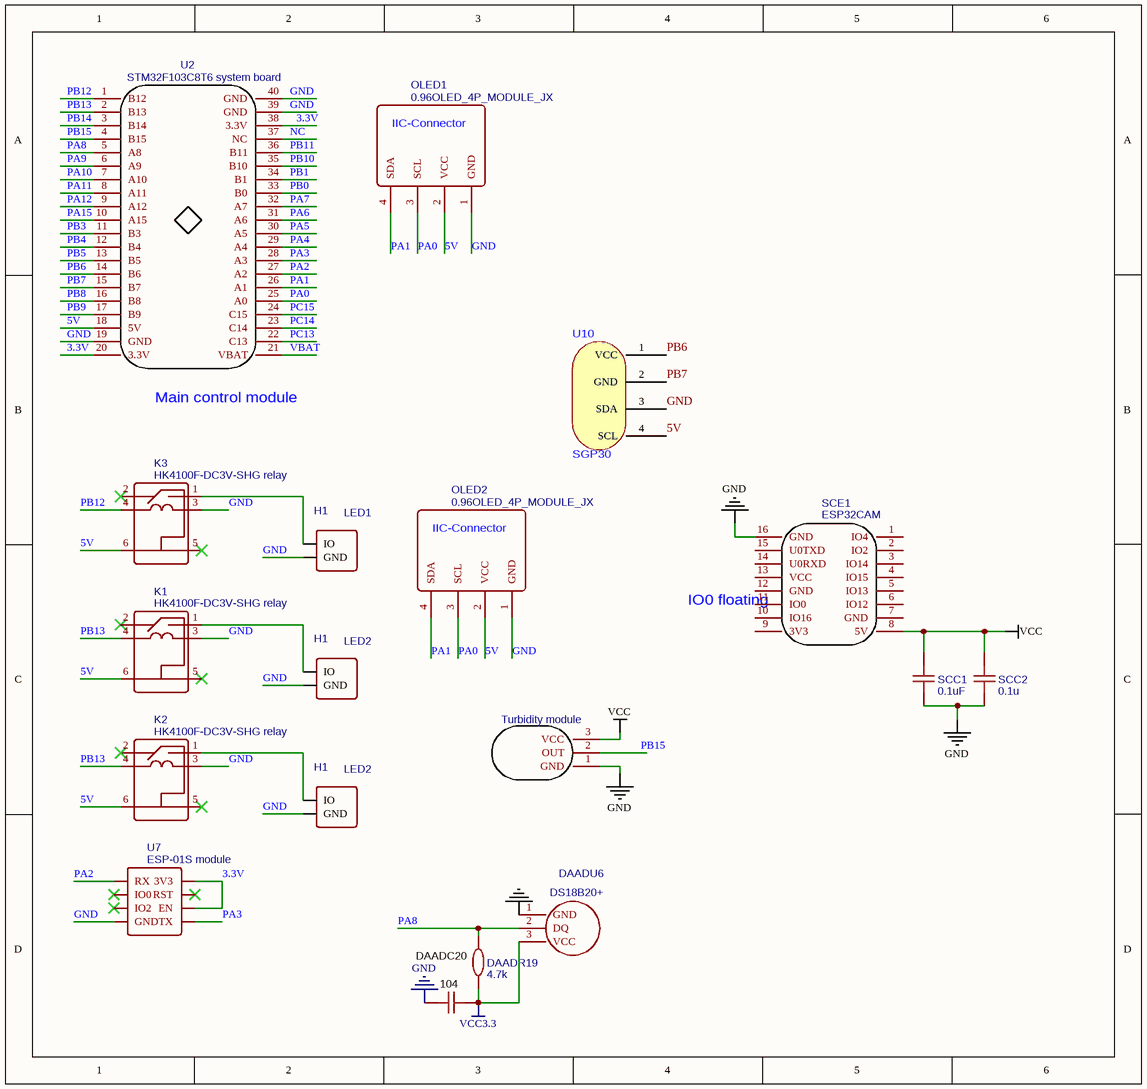
[diagram p0: MISC82816-7.schdoc]
# Altium project MISC82816-7.PrjPcb
1 sheet, 18 parts. Net scope: global (net labels, ports and power ports of the same name join across sheets).
Board file: MISC82816.PcbDoc

## Sheet MISC82816-7.schdoc
size 213 x 203 mm

### Parts
DAADC20  104  [C0603]
DAADR19  4.7k  [AXIAL-0.3]
DAADU6  DS18B20+  [DS18B20]
K1  HK4100F-DC3V-SHG relay  [HK4100F]
K2  HK4100F-DC3V-SHG relay  [HK4100F]
K3  HK4100F-DC3V-SHG relay  [HK4100F]
OLED1  0.96OLED_4P_MODULE_JX  [0.96OLED_4P]
OLED2  0.96OLED_4P_MODULE_JX  [0.96OLED_4P]
SCC1  0.1uF  [C0603]
SCC2  0.1u  [C0603]
SCE1  ESP32CAM  [ESP32CAM]
U1  DC motor terminal  [HDR1X2]  (value not drawn)
U2  STM32F103C8T6 system board  [STM32核心板]
U3  DC motor terminal  [HDR1X2]  (value not drawn)
U5  DC motor terminal  [hdr1x2]  (value not drawn)
U6  Turbidity module  [HDR1X3]
U7  ESP-01S module  [WIFI]
U10  SGP30  [SGP30]

### Nets
GND: DAADC20.1 DAADU6.1(GND) K1.3 K2.3 K3.3 OLED1.1(GND) OLED2.1(GND) SCC1.1 SCC2.1 SCE1.16(GND) U1.2(GND) U2.19(GND) U2.39(GND) U2.40(GND) U3.2(GND) U5.2(GND) U6.1(GND) U7.5(GND) U10.3(SDA)
VCC: SCC1.2 SCC2.2 SCE1.8(5V) U6.3(VCC)
VCC3.3: DAADC20.2 DAADR19.1 DAADU6.3(VCC)
3.3V: U2.20(3.3V) U2.38(3.3V) U7.1(3V3) U7.3(EN)
5V: K1.6 K2.6 K3.6 OLED1.2(VCC) OLED2.2(VCC) U2.18(5V) U10.4(SCL)
NC: U2.37(NC)
PA0: OLED1.3(SCL) OLED2.3(SCL) U2.25(A0)
PA1: OLED1.4(SDA) OLED2.4(SDA) U2.26(A1)
PA2: U2.27(A2) U7.8(RX)
PA3: U2.28(A3) U7.4(TX)
PA4: U2.29(A4)
PA5: U2.30(A5)
PA6: U2.31(A6)
PA7: U2.32(A7)
PA8: DAADR19.2 DAADU6.2(DQ) U2.5(A8)
PA9: U2.6(A9)
PA10: U2.7(A10)
PA11: U2.8(A11)
PA12: U2.9(A12)
PA15: U2.10(A15)
PB0: U2.33(B0)
PB1: U2.34(B1)
PB3: U2.11(B3)
PB4: U2.12(B4)
PB5: U2.13(B5)
PB6: U2.14(B6) U10.1(VCC)
PB7: U2.15(B7) U10.2(GND)
PB8: U2.16(B8)
PB9: U2.17(B9)
PB10: U2.35(B10)
PB11: U2.36(B11)
PB12: K3.4 U2.1(B12)
PB13: K1.4 K2.4 U2.2(B13)
PB14: U2.3(B14)
PB15: U2.4(B15) U6.2(OUT)
PC13: U2.22(C13)
PC14: U2.23(C14)
PC15: U2.24(C15)
VBAT: U2.21(VBAT)
NetK1_1: K1.1 U1.1(IO)
NetK2_1: K2.1 U3.1(IO)
NetK3_1: K3.1 U5.1(IO)

Not connected (* = marked no-connect by the designer): K1 2* 5*; K2 2* 5*; K3 2* 5*; SCE1 1(IO4) 2(IO2) 3(IO14) 4(IO15) 5(IO13) 6(IO12) 7(GND) 9(3V3) 10(IO16) 11(IO0) 12(GND) 13(VCC) 14(U0RXD) 15(U0TXD); U7 2(RST)* 6(IO2)* 7(IO0)*

### Notes on the sheet
- (near U2) Main control module
- (near SCE1) IO0 floating

### Library data of the parts
DAADC20 = 104: nameAlias: Value(F); Contributor: LCEDA_Lib; spicePre: C; spiceSymbolName: C_0201_US
DAADR19 = 4.7k: nameAlias: Value(Ω); Manufacturer Part: ?; spicePre: R; spiceSymbolName: Res_AXIAL-0.3(1/8W)_EU
DAADU6 = DS18B20+: Manufacturer: MAXIM; Supplier: LCSC; Manufacturer Part: DS18B20+; image: C9753.jpg; spicePre: U; Supplier Part: C9753
K1-K3 = HK4100F-DC3V-SHG继电器: Manufacturer: Ningbo Keke New Era Appliance; Contributor: LCSC; Supplier: LCSC; Supplier Part: C98931; Manufacturer Part: HK4100F-DC3V-SHG; spicePre: K; spiceSymbolName: HK4100F-DC3V-SHG relay
OLED1 OLED2 = 0.96OLED_4P_MODULE_JX: Manufacturer: null; Contributor: LCSC; Supplier: LCSC; Supplier Part: C9900004566; Manufacturer Part: 0.96OLED_4P_MODULE_JX; JLCPCB Part Class: Extended Part; link: https://so.szlcsc.com/global.html?k=C9900004566&ref=editor; spicePre: O; spiceSymbolName: 0.96OLED_4P_MODULE_JX
SCC1 = 0.1uF: nameAlias: Value(F); Contributor: LCEDA_Lib; spicePre: C; spiceSymbolName: C_0603_US
SCC2 = 0.1u: nameAlias: Value(F); Contributor: LCEDA_Lib; spicePre: C; spiceSymbolName: C_0603_US
SCE1 = ESP32CAM: Contributor: test1test; spicePre: M; spiceSymbolName: ESP32CAM COPY
U1 U3 U5 = 直流电机端子: spicePre: U; spiceSymbolName: DC motor terminal
U2 = STM32F103C8T6系统板: Contributor: wwwxxb; spicePre: U; spiceSymbolName: STM32F103C8T6 system board
U6 = 浑浊度模块: Contributor: V541; spicePre: U; spiceSymbolName: DHT11
U7 = ESP-01S模块: Contributor: PERSON_A; spicePre: U; spiceSymbolName: ESP-01S module